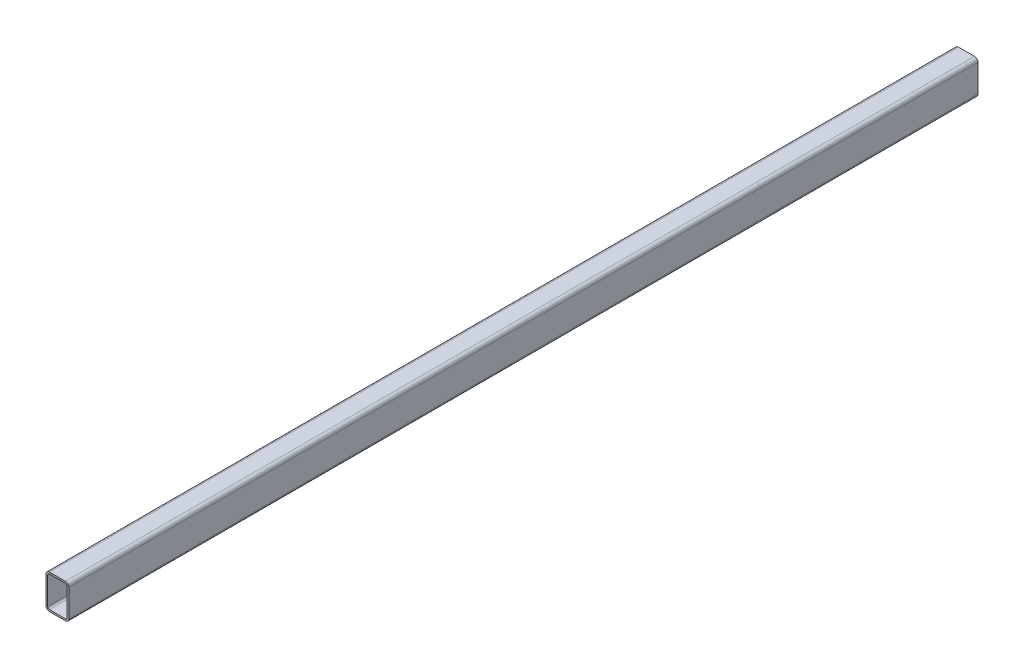
SolidWorks part; units mm, degrees
material "普通碳钢"
ref_plane "Front Plane" through (0, 0, 0) normal (0, 0, 1) x (1, 0, 0)
ref_plane "Top Plane" through (0, 0, 0) normal (0, 1, 0) x (1, 0, 0)
ref_plane "Right Plane" through (0, 0, 0) normal (1, 0, 0) x (0, 0, -1)
other "Configuration Table"
sketch "Sketch1" plane through (0, 0, 0) normal (0, 1, 0) x (1, 0, 0)
  line L0 (0, 0) -> (0, 1590)
  dimension "D1" = 1590
other "Gb/6728-1986 rectangular hollow section 060 X 40 X 3"
ref_plane "Plane1" through (0, 0, 0) normal (0, 0, -1) x (-1, 0, 0)
sketch "Sketch14" plane through (0, 0, 0) normal (0, 0, -1) x (-1, 0, 0)
  line L0 (-14, -27) -> (14, -27)
  line L1 (-17, -24) -> (-17, 24)
  line L2 (14, 27) -> (-14, 27)
  line L3 (17, 24) -> (17, -24)
  line L4 (-14, -30) -> (14, -30)
  line L5 (-20, -24) -> (-20, 24)
  line L6 (14, 30) -> (-14, 30)
  line L7 (20, 24) -> (20, -24)
  arc A0 (20, 24) -> (14, 30) centre (14, 24) ccw
  arc A1 (14, -30) -> (20, -24) centre (14, -24) ccw
  arc A2 (-20, -24) -> (-14, -30) centre (-14, -24) ccw
  arc A3 (-14, 30) -> (-20, 24) centre (-14, 24) ccw
  arc A4 (-14, 27) -> (-17, 24) centre (-14, 24) ccw
  arc A5 (17, 24) -> (14, 27) centre (14, 24) ccw
  arc A6 (14, -27) -> (17, -24) centre (14, -24) ccw
  arc A7 (-17, -24) -> (-14, -27) centre (-14, -24) ccw
  point P0 (0, 30)
  point P1 (20, 0)
  point P2 (0, -30)
  point P3 (-20, 0)
  point P4 (-20, 30)
  point P5 (20, 30)
  point P6 (20, -30)
  point P7 (-20, -30)
  point P8 (0, 0)
  point P33 (0, 0)
  dimension "D1" = 6
  dimension "Thickness" = 3
  dimension "V_leg" = 60
  dimension "H_leg" = 40
sketch "Sketch2" plane through (-20, 0, 0) normal (-1, 0, 0) x (0, 0, 1)
  line L0 (-1590, 0) -> (0, 0) construction
  line L1 (-1590, -24) -> (-1590, 24) construction
  circle A0 centre (-800, 0) radius 15
  dimension "D1" = 30
  dimension "D2" = 790
extrude "Cut-Extrude1" [suppressed] cut sketch "Sketch2" against normal through all
sketch "Sketch3" [suppressed] plane through (-20, 0, 0) normal (-1, 0, 0) x (0, 0, 1)
  line L0 (-1590, 24) -> (0, 24) construction
  line L1 (-860, -24) -> (-740, -24)
  line L2 (-860, -24) -> (-860, 24)
  line L3 (-860, 24) -> (-740, 24)
  line L4 (-740, -24) -> (-740, 24)
  line L5 (-860, -24) -> (-740, 24) construction
  line L6 (-860, 24) -> (-740, -24) construction
  circle A0 centre (-800, 0) radius 15
  point P0 (-800, 0)
  dimension "D2" = 30
  dimension "D1" = 120
